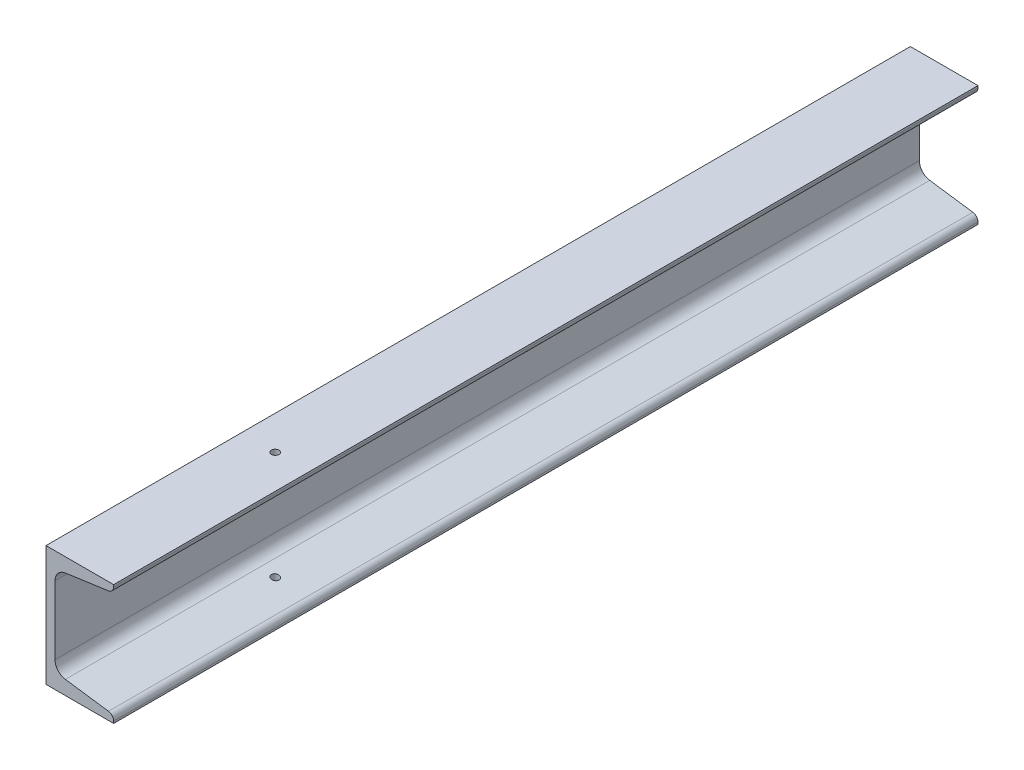
SolidWorks part; units mm, degrees
ref_plane "前视基准面" through (0, 0, 0) normal (0, 0, 1) x (1, 0, 0)
ref_plane "上视基准面" through (0, 0, 0) normal (0, 1, 0) x (1, 0, 0)
ref_plane "右视基准面" through (0, 0, 0) normal (1, 0, 0) x (0, 0, -1)
sketch "草图1" plane through (0, 0, 0) normal (0, 0, 1) x (1, 0, 0)
  line L0 (0, 0) -> (-45, 0)
  line L1 (-45, 0) -> (-45, -80)
  line L2 (-45, -80) -> (0, -80)
  line L3 (0, -80) -> (0, -78.6393)
  line L4 (-3.4433, -74.6782) -> (-32.1134, -70.6489)
  line L5 (-39, -62.7268) -> (-39, -17.2732)
  line L6 (-32.1134, -9.3511) -> (-3.4433, -5.3218)
  line L7 (0, -1.3607) -> (0, 0)
  line L8 (-22.5, -72) -> (-22.5, -80) construction
  arc A0 (-32.1134, -70.6489) -> (-39, -62.7268) centre (-31, -62.7268) cw
  arc A1 (-39, -17.2732) -> (-32.1134, -9.3511) centre (-31, -17.2732) cw
  arc A2 (0, -78.6393) -> (-3.4433, -74.6782) centre (-4, -78.6393) ccw
  arc A3 (-3.4433, -5.3218) -> (0, -1.3607) centre (-4, -1.3607) ccw
  point P11 (0, -74.2141)
  dimension "D8" = 8
  dimension "D9" = 4
  dimension "D1" = 80
  dimension "D2" = 45
  dimension "D3" = 6
  dimension "D4" = 22.5
  dimension "D5" = 8
  dimension "D6" = 8
  dimension "D7" = 8
extrude "凸台-拉伸1" add sketch "草图1" along normal blind 575
sketch "草图2" plane through (0, -80, 0) normal (0, -1, 0) x (1, 0, 0)
  line L0 (0, 575) -> (0, 0) construction
  line L1 (-45, 575) -> (0, 575) construction
  circle A0 centre (-22.5, 445) radius 2
  dimension "D1" = 22.5
  dimension "D3" = 4
  dimension "D2" = 130
hole_wizard "M6 螺纹孔1" positions "草图3" profile "草图5" tap size "M6" standard "ISO" end condition through all
sketch "草图3" plane through (0, -80, 0) normal (0, -1, 0) x (-1, 0, 0)
  point P0 (22.5, -445)
sketch "草图5" plane through (-22.5, -80, 445) normal (1, 0, 0) x (0, 0, -1)
  line L0 (0, 0) -> (0, 80)
  line L1 (0, 80) -> (2.5, 80)
  line L2 (2.5, 80) -> (2.5, 0)
  line L5 (2.5, 0) -> (0, 0)
  line L11 (0, -6.35) -> (0, 107.95) construction
  dimension "通孔螺纹孔钻头直径" = 5
  dimension "通孔螺纹孔钻头深度" = 80
cosmetic thread "孔螺蚊线1" parameters "D2"=6
